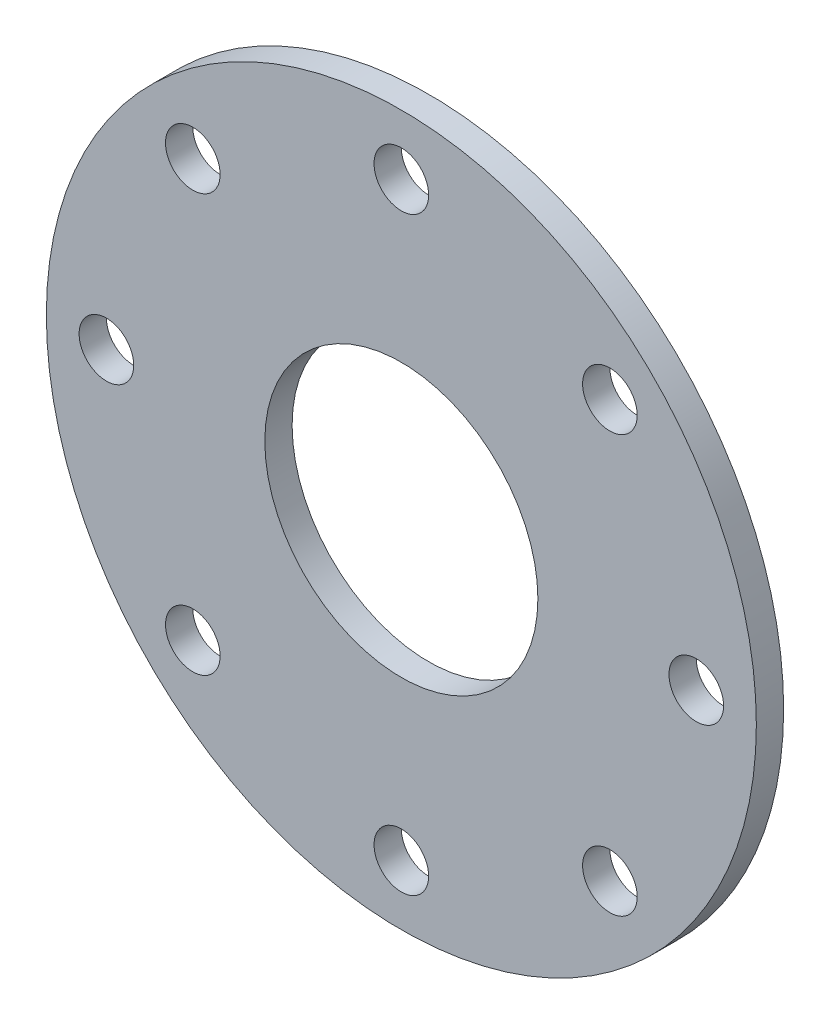
from build123d import *

# Parameters (mm, degrees)
SKETCH_1_R          = 130
SKETCH_1_R_2        = 10
EXTRUDE_1_DEPTH     = 5
SKETCH_2_R          = 50
CUT_EXTRUDE_1_DEPTH = 10


with BuildPart() as part:
    # 草图1 → 凸台-拉伸1 (new, symmetric)
    with BuildSketch(Plane.XY):
        Circle(SKETCH_1_R)
        with Locations((0, 108)):
            Circle(SKETCH_1_R_2, mode=Mode.SUBTRACT)
        with Locations((76.367532368, 76.367532368)):
            Circle(SKETCH_1_R_2, mode=Mode.SUBTRACT)
        with Locations((108, 0)):
            Circle(SKETCH_1_R_2, mode=Mode.SUBTRACT)
        with Locations((76.367532368, -76.367532368)):
            Circle(SKETCH_1_R_2, mode=Mode.SUBTRACT)
        with Locations((0, -108)):
            Circle(SKETCH_1_R_2, mode=Mode.SUBTRACT)
        with Locations((-76.367532368, -76.367532368)):
            Circle(SKETCH_1_R_2, mode=Mode.SUBTRACT)
        with Locations((-108, 0)):
            Circle(SKETCH_1_R_2, mode=Mode.SUBTRACT)
        with Locations((-76.367532368, 76.367532368)):
            Circle(SKETCH_1_R_2, mode=Mode.SUBTRACT)
    extrude(amount=EXTRUDE_1_DEPTH, both=True)

    # 草图2 → 切除-拉伸1 (cut)
    with BuildSketch(Plane.XY.offset(5)):
        Circle(SKETCH_2_R)
    extrude(amount=-CUT_EXTRUDE_1_DEPTH, mode=Mode.SUBTRACT)


solid = part.part
